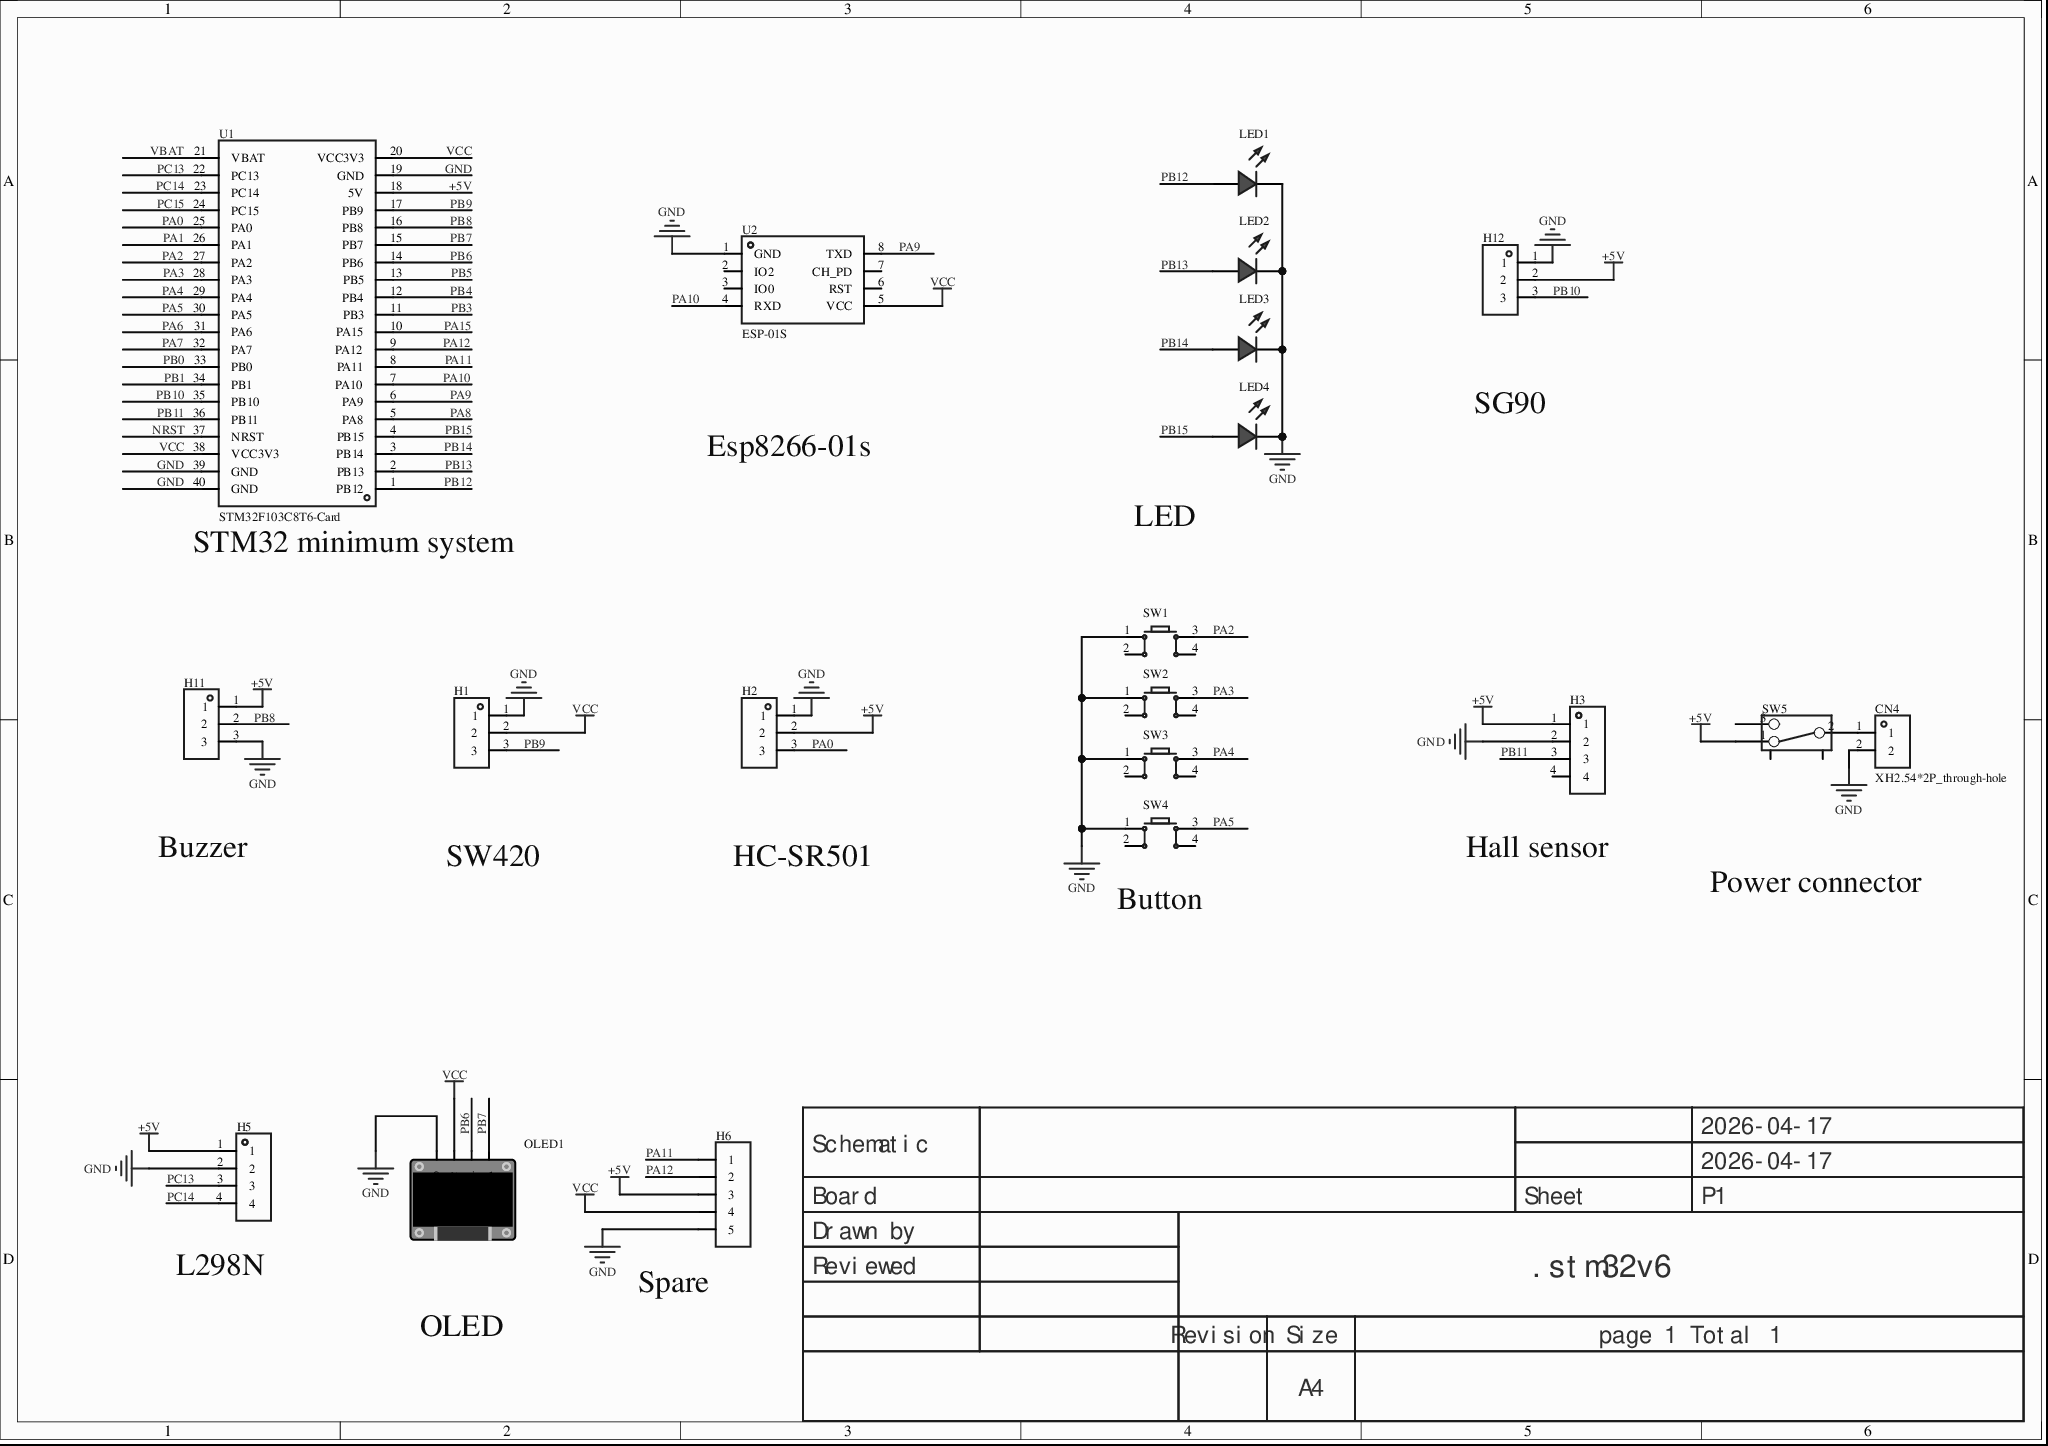
[diagram p0: MISC51767-3.schdoc]
# Altium project MISC51767-2.PrjPcb
1 sheet, 20 parts. Net scope: global (net labels, ports and power ports of the same name join across sheets).
Board file: MISC51767.pcbdoc

## Sheet MISC51767-3.schdoc
size 297 x 209 mm; Version: V1.0; @Project Name: MISC51767; @Page Count: 1; @Update Date: 2026-04-17; @Create Date: 2026-04-17; @Schematic Name: MISC51767; @Page No: 1; @Create Time: 23:22:16; @Update Time: 17:32:40; @Board Name: MISC51767

### Parts
CN4  XH2.54*2P_through-hole  [CONN-TH_2P-P2.50-XH2.54-2P]
H1  (no value)  [HDR-TH_3P-P2.54-V-F]
H2  (no value)  [HDR-TH_3P-P2.54-V-F]
H3  (no value)  [HDR-TH_4P-P2.54-V-F]
H5  (no value)  [HDR-TH_4P-P2.54-V-F]
H6  (no value)  [HDR-TH_5P-P2.54-V-F]
H11  (no value)  [HDR-TH_3P-P2.54-V-F]
H12  (no value)  [HDR-TH_3P-P2.54-V-F]
LED1  (no value)  [LED-TH_5mm]
LED2  (no value)  [LED-TH_5mm]
LED3  (no value)  [LED-TH_5mm]
LED4  (no value)  [LED-TH_5mm]
OLED1  (no value)  [0.96OLED_4P]
SW1  (no value)  [SW-TH_4P-L6.0-W6.0-P4.50-LS6.5]
SW2  (no value)  [SW-TH_4P-L6.0-W6.0-P4.50-LS6.5]
SW3  (no value)  [SW-TH_4P-L6.0-W6.0-P4.50-LS6.5]
SW4  (no value)  [SW-TH_4P-L6.0-W6.0-P4.50-LS6.5]
SW5  (no value)  [拨动开关]
U1  STM32F103C8T6-Card  [CONN-TH_L53.3-W22.9_STM32F103C8T6-CARD]
U2  ESP-01S  [WIFIM-TH_ESP-01S]

### Nets
+5V: H2.2 H3.1 H5.1 H6.3 H11.1 H12.2 SW5.1 U1.18(5V)
GND: CN4.2 H1.1 H2.1 H3.2 H5.2 H6.5 H11.3 H12.1 LED1.2(A) LED2.2(A) LED3.2(A) LED4.2(A) OLED1.1(GND) SW1.1 SW2.1 SW3.1 SW4.1 U1.19(GND) U1.39(GND) U1.40(GND) U2.1(GND)
VCC: H1.2 H6.4 OLED1.2(VCC) U1.20(VCC3V3) U1.38(VCC3V3) U2.5(VCC)
NRST: U1.37(NRST)
PA0: H2.3 U1.25(PA0)
PA1: U1.26(PA1)
PA2: SW1.3 U1.27(PA2)
PA3: SW2.3 U1.28(PA3)
PA4: SW3.3 U1.29(PA4)
PA5: SW4.3 U1.30(PA5)
PA6: U1.31(PA6)
PA7: U1.32(PA7)
PA8: U1.5(PA8)
PA9: U1.6(PA9) U2.8(TXD)
PA10: U1.7(PA10) U2.4(RXD)
PA11: H6.1 U1.8(PA11)
PA12: H6.2 U1.9(PA12)
PA15: U1.10(PA15)
PB0: U1.33(PB0)
PB1: U1.34(PB1)
PB3: U1.11(PB3)
PB4: U1.12(PB4)
PB5: U1.13(PB5)
PB6: OLED1.3(SCL) U1.14(PB6)
PB7: OLED1.4(SDA) U1.15(PB7)
PB8: H11.2 U1.16(PB8)
PB9: H1.3 U1.17(PB9)
PB10: H12.3 U1.35(PB10)
PB11: H3.3 U1.36(PB11)
PB12: LED1.1(C) U1.1(PB12)
PB13: LED2.1(C) U1.2(PB13)
PB14: LED3.1(C) U1.3(PB14)
PB15: LED4.1(C) U1.4(PB15)
PC13: H5.3 U1.22(PC13)
PC14: H5.4 U1.23(PC14)
PC15: U1.24(PC15)
VBAT: U1.21(VBAT)
NetCN4_1: CN4.1 SW5.2

Not connected (* = marked no-connect by the designer): H3 4; SW1 2 4; SW2 2 4; SW3 2 4; SW4 2 4; SW5 3 4 5; U2 2(IO2)* 3(IO0)* 6(RST)* 7(CH_PD)*

### Notes on the sheet
- 串口：
  ESP8266-01s  		PA10，PA9 	(串口1）
  GPIO:
  LED灯	PB12、PB13、PB14、PB15、
  SG90 PB10  5V电源
  蜂鸣器  PB8  5V电源 GND
  SW420振动传感器 PB9 3.3v GND
  HC-SR501人体红外传感器 PA0  5V电源 GND
  按键：	PA2，PA3，PA4，PA5
  霍尔传感器 PB11 5V电源 GND
  L298N电机驱动模块  PC13 PC14 5V供电 GND
  IIC:
  0.96英寸OLED显示屏	PB6，PB7
- SG90
- Esp8266-01s
- (near U1) STM32 minimum system
- LED
- Buzzer
- SW420
- HC-SR501
- (near H3) Hall sensor
- (near SW4) Button
- Power connector
- (near H5) L298N
- (near H6) Spare
- OLED
- 2026-04-17
- Schematic
- Board
- Sheet
- P1
- Drawn by
- Reviewed
- .stm32v6
- Revision
- Size
- A4
- page 1 Total 1

### Library data of the parts
CN4 = XH2.54*2P_直插: 3D Model: 325c595e30db4df8abe76612dd40b0fa0819f05c4eef4c71ace90d822a990e87; 3D Model Transform: 295.275,228.346,0,180,0,0,-0.002,-20.079,-137.795; AddInBom: yes; Symbol: XH2.54*2P_through-hole; Device: XH2.54*2P_through-hole; LCSC Part Name: XH2.54*2P_直插; Supplier Part: C9900008615; Manufacturer Part: XH2.54*2P_直插; Supplier Footprint: XH2.54_2P; JLCPCB Part Class: Extended Part; Supplier: LCSC; ConvertToPcb: yes; FootprintName: CONN-TH_2P-P2.50-XH2.54-2P; ModelName: CONN-TH_2P-P2.50-XH2.54-2P
H1 H2 H11 H12 = HDR-F_2.54_1x3P: Symbol: PM254V-11-03-H85; 3D Model: f3b3cc5aae9641bf9e56fc160cef875b; 3D Model Transform: 299.9994,100,0,0,0,0,0,0,-118.11; ConvertToPcb: yes; ModelName: HDR2.54-F-LI-1X3P; Device: HDR-F_2.54_1x3P; Supplier Part: C541850; Supplier Footprint: 插件; AddInBom: yes; FootprintName: HDR-TH_3P-P2.54-V-F
H3 H5 = HDR-F_2.54_1x4P: Symbol: 2.54-1*4P female; ConvertToPcb: yes; ModelId: d187812051054f85879fcaa51a310d8e0819f05c4eef4c71ace90d822a990e87; ModelTransform: 419.6842,98.464,0,0,0,0,0,0,-118.11; Device: HDR-F_2.54_1x4P; AddInBom: yes; SupplierPart: C2718488; Supplier Footprint: 插件; FootprintName: HDR-TH_4P-P2.54-V-F; ModelName: HDR-TH_4P-P2.54-V-F
H6 = HDR-F_2.54_1x5P: Symbol: Header-Female-2.54_1x5; ConvertToPcb: yes; ModelId: f49cb6116a3d45e5a64915bf3e00773f; ModelTransform: 519.684,98.464,0,0,0,0,0,0,-124.016; Device: HDR-F_2.54_1x5P; AddInBom: yes; SupplierPart: C50950; Supplier Footprint: 插件; FootprintName: HDR-TH_5P-P2.54-V-F; ModelName: HDR-TH_5P-P2.54-V-F
LED1-LED4 = LED_TH-R_5mm: ConvertToPcb: yes; ModelId: fe9cea1bdf7642cd8d9a5077ed0e2b580819f05c4eef4c71ace90d822a990e87; ModelName: LED-TH_BD5.9-P2.54-RD_RED; ModelTransform: 222.16,238.98,581.81,180,0,0,-6,0,-220; Symbol: LED_TH-R; Device: LED_TH-R_5mm; AddInBom: yes; FootprintName: LED-TH_5mm; Supplier Footprint: 插件
OLED1 = 0.96OLED模块_4P: Symbol: 0.96OLED module_4P; ConvertToPcb: yes; ModelId: 79c000fdb68d45a296c2e9bedf4f9055; ModelTransform: 1393.69792,1318.895,0,0,0,0,0,-560.079,-137.795; Device: 0.96OLED module_4P; AddInBom: yes; FootprintName: 0.96OLED_4P; Supplier Footprint: 插件; ModelName: 0.96OLED_4P
SW1-SW4 = Key_TH_6x6x6: 触点电流:50mA;额定电压(DC):12V;绝缘电阻:100MΩ;电路结构:单刀单掷;安装方式:直插;按钮形状:圆形按钮;按钮/盖帽颜色:黑色;作用力:260gf@±30gf;工作温度:-25℃~+70℃;引脚样式:PC引脚;开关长度:6mm;开关宽度:6mm;开关高度:6mm;带支架:否;; Symbol: Tact switch; AddInBom: yes; ModelId: 20eee248bc684ccd8cbdbb1d0d91ec6f0819f05c4eef4c71ace90d822a990e87; ModelName: SW-TH_4P-L6.0-W6.0-H5.0-LS6.5-P4.50; ModelTransform: 236.22,323.03,0,90,0,0,0,0,-137.795; Device: Key_TH_6x6x6; ConvertToPcb: yes; FootprintName: SW-TH_4P-L6.0-W6.0-P4.50-LS6.5; Supplier Footprint: 插件
SW5 = 拨动开关_正: Symbol: Toggle switch; Device: Toggle switch_upright; ConvertToPcb: yes; ModelId: 4321fe59a4074cbfb4989553f297c68f0819f05c4eef4c71ace90d822a990e87; ModelName: SW-TH_SS-12D02-VG4; ModelTransform: 370.09,208.7,472.35,0,0,0,0,0,-110; AddInBom: yes; Supplier Footprint: 插件; FootprintName: Toggle switch
U1 = STM32F103C8T6-Card: AddInBom: yes; Symbol: STM32F103C8T6-CARD; Device: STM32F103C8T6-Card; LCSC Part Name: STM32F103C8T6-Card; SupplierPart: C9900077949; ManufacturerPart: STM32F103C8T6-Card; Supplier Footprint: 插件; Supplier: LCSC; ConvertToPcb: yes; FootprintName: CONN-TH_L53.3-W22.9_STM32F103C8T6-CARD
U2 = ESP-01S_C111009: AddInBom: yes; ModelId: eb7175da78ae48b3b1568cfe3027405f0819f05c4eef4c71ace90d822a990e87; ModelTransform: 582.676,976.37608,0,0,0,0,0,388.346,-118.11; Symbol: ESP-01S; Device: ESP-01S_C111009; LCSC Part Name: ESP-01S; SupplierPart: C111009; ManufacturerPart: ESP-01S; Supplier Footprint: -; JLCPCB Part Class: Extended Part; Supplier: LCSC; ConvertToPcb: yes; FootprintName: WIFIM-TH_ESP-01S; ModelName: WIFIM-TH_ESP-01S